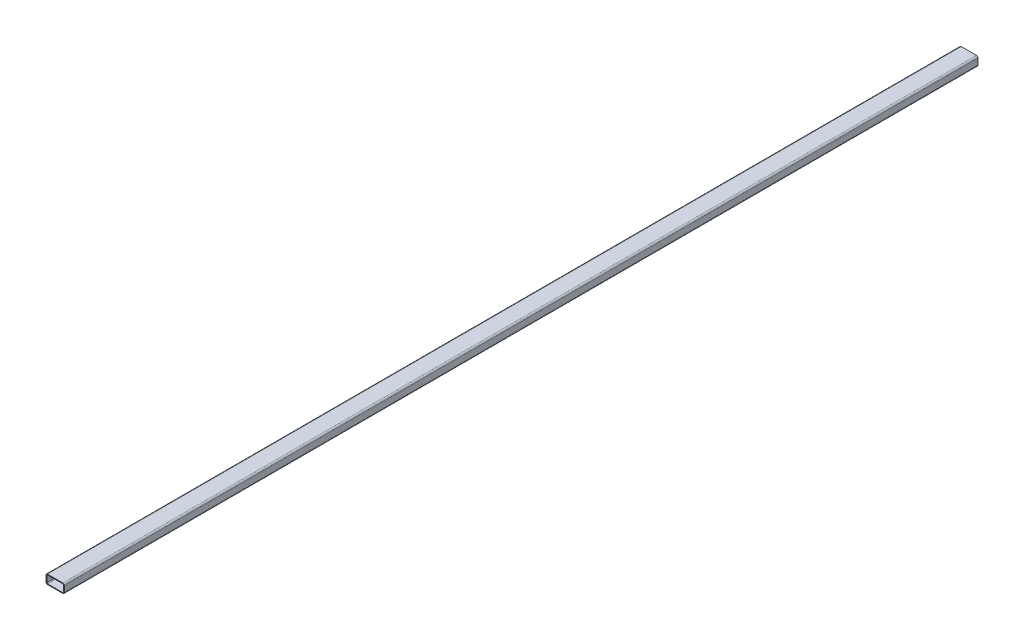
from build123d import *

# Parameters (mm, degrees)
BOSS_EXTRUDE1_DEPTH = 6000


with BuildPart() as part:
    # Sketch1 → Boss-Extrude1 (new body)
    with BuildSketch(Plane.XY):
        with BuildLine():
            Line((10, 0), (110, 0))
            ThreePointArc((110, 0), (117.071067812, 2.928932188), (120, 10))
            Line((120, 10), (120, 50))
            ThreePointArc((120, 50), (117.071067812, 57.071067812), (110, 60))
            Line((110, 60), (10, 60))
            ThreePointArc((10, 60), (2.928932188, 57.071067812), (0, 50))
            Line((0, 50), (0, 10))
            ThreePointArc((0, 10), (2.928932188, 2.928932188), (10, 0))
        make_face()
        with BuildLine():
            Line((10, 55), (110, 55))
            ThreePointArc((110, 55), (113.535533906, 53.535533906), (115, 50))
            Line((115, 50), (115, 10))
            ThreePointArc((115, 10), (113.535533906, 6.464466094), (110, 5))
            Line((110, 5), (10, 5))
            ThreePointArc((10, 5), (6.464466094, 6.464466094), (5, 10))
            Line((5, 10), (5, 50))
            ThreePointArc((5, 50), (6.464466094, 53.535533906), (10, 55))
        make_face(mode=Mode.SUBTRACT)
    extrude(amount=BOSS_EXTRUDE1_DEPTH)


solid = part.part
